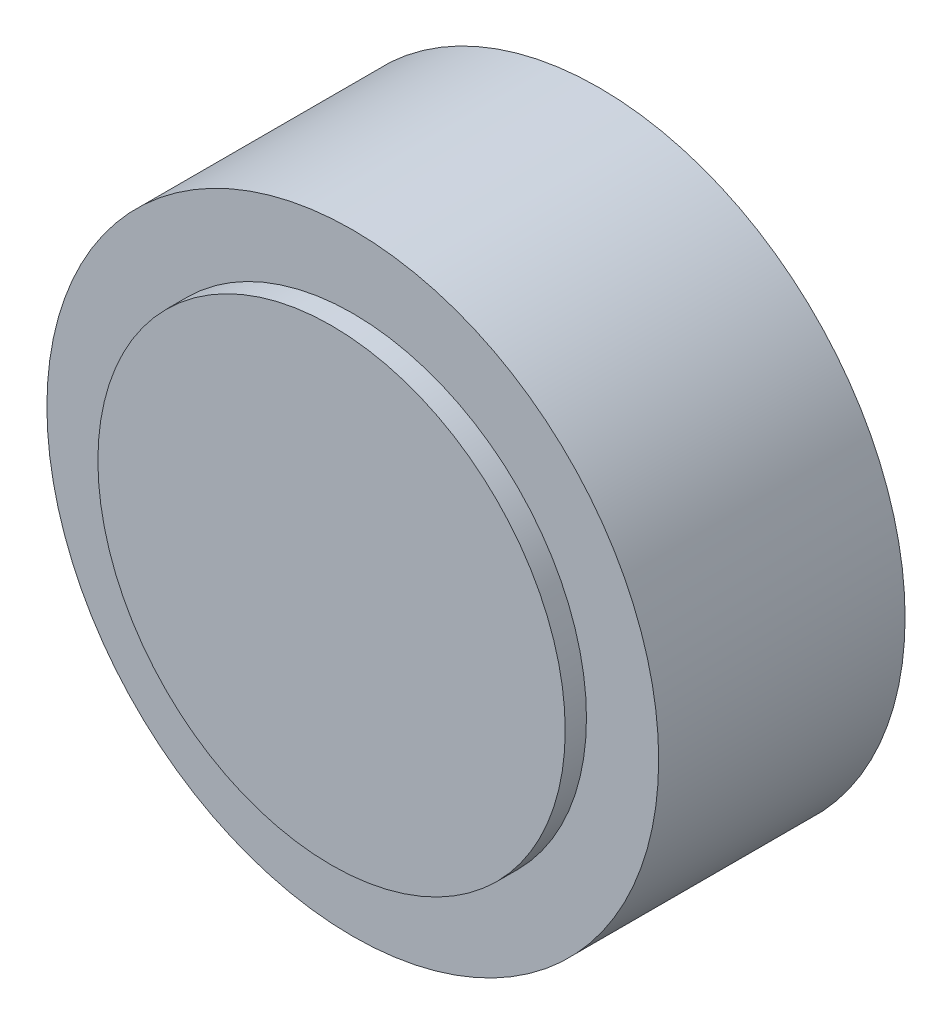
from build123d import *

# Parameters (mm, degrees)
SKETCH1_R           = 72
BOSS_EXTRUDE1_DEPTH = 58
SKETCH2_R           = 55
BOSS_EXTRUDE2_DEPTH = 5


with BuildPart() as part:
    # Sketch1 → Boss-Extrude1 (new body)
    with BuildSketch(Plane.XY):
        with Locations(Location((0, 0, 0), (0, 0, 180))):
            Circle(SKETCH1_R)
    extrude(amount=BOSS_EXTRUDE1_DEPTH)

    # Sketch2 → Boss-Extrude2 (add)
    with BuildSketch(Plane.XY.offset(58)):
        Circle(SKETCH2_R)
    extrude(amount=BOSS_EXTRUDE2_DEPTH)


solid = part.part
